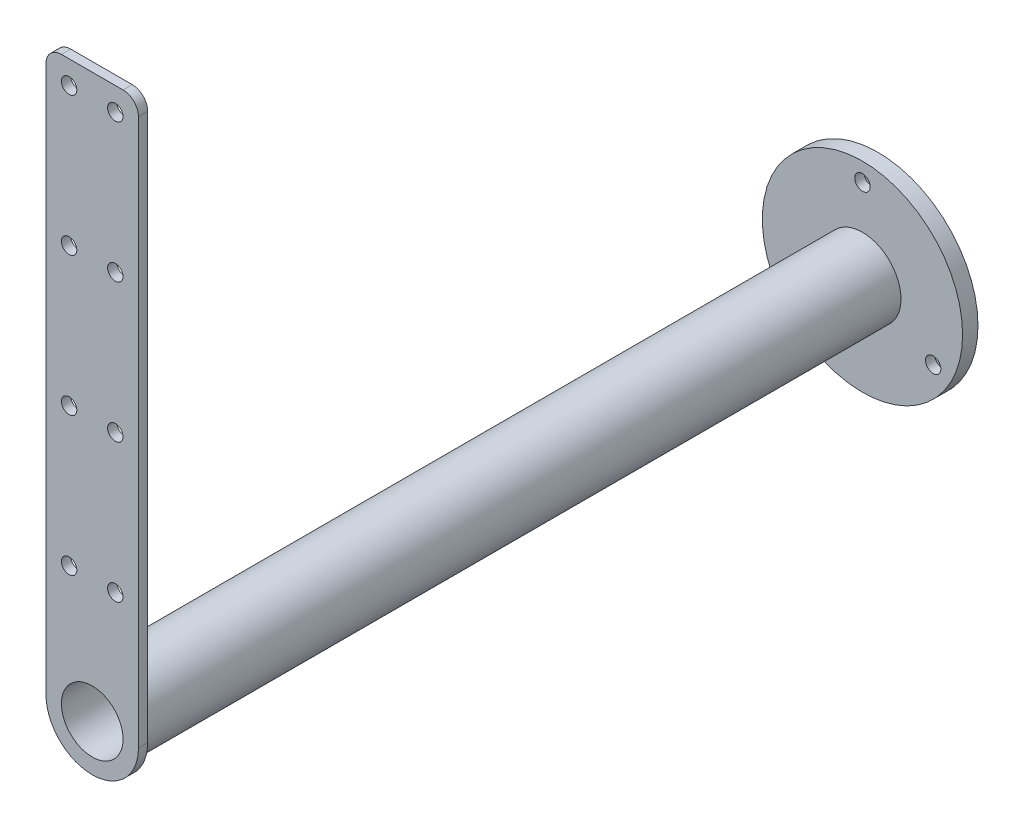
SolidWorks part; units mm, degrees
ref_plane "Front Plane" through (0, 0, 0) normal (0, 0, 1) x (1, 0, 0)
ref_plane "Top Plane" through (0, 0, 0) normal (0, 1, 0) x (1, 0, 0)
ref_plane "Right Plane" through (0, 0, 0) normal (1, 0, 0) x (0, 0, -1)
sketch "Sketch1" plane through (0, 0, 0) normal (0, 0, 1) x (1, 0, 0)
  circle A0 centre (0, 0) radius 65
  circle A1 centre (0, 0) radius 20
  dimension "D1" = 130
  dimension "D2" = 40
extrude "Boss-Extrude1" add sketch "Sketch1" along normal blind 10
sketch "Sketch2" plane through (0, 0, 10) normal (0, 0, 1) x (1, 0, 0)
  circle A0 centre (0, 0) radius 25
  circle A1 centre (0, 0) radius 20 construction
  circle A2 centre (0, 0) radius 20
  dimension "D1" = 50
extrude "Boss-Extrude2" add sketch "Sketch2" along normal blind 494
sketch "Sketch3" plane through (0, 0, 504) normal (0, 0, 1) x (1, 0, 0)
  line L0 (-30, 0) -> (-30, 365)
  line L1 (-30, 365) -> (30, 365)
  line L2 (30, 365) -> (30, 0)
  arc A0 (-30, 0) -> (30, 0) centre (0, 0) ccw
  circle A1 centre (0, 0) radius 20
  dimension "D1" = 60
  dimension "D2" = 365
extrude "Boss-Extrude3" add sketch "Sketch3" along normal blind 6
fillet "Fillet1" radius 10 2 edges at (-30, 365, 507) (30, 365, 507)
sketch "Sketch4" plane through (0, 0, 510) normal (0, 0, 1) x (1, 0, 0)
  line L0 (0, 365) -> (0, 386.1458) construction
  line L1 (20, 365) -> (-20, 365) construction
  circle A0 centre (-15, 350) radius 5
  circle A1 centre (15, 350) radius 5
  circle A2 centre (-15, 260) radius 5
  circle A3 centre (15, 260) radius 5
  circle A4 centre (-15, 170) radius 5
  circle A5 centre (15, 170) radius 5
  circle A6 centre (-15, 80) radius 5
  circle A7 centre (15, 80) radius 5
  dimension "D4" = 10
  dimension "D1" = 30
  dimension "D2" = 15
  dimension "D3" = 15
  dimension "D5" = 4
extrude "Cut-Extrude1" cut sketch "Sketch4" against normal blind 6
sketch "Sketch5" plane through (0, 0, 10) normal (0, 0, 1) x (1, 0, 0)
  circle A0 centre (0, 0) radius 53 construction
  circle A1 centre (0, 53) radius 5
  circle A2 centre (45.8993, -26.5) radius 5
  circle A3 centre (-45.8993, -26.5) radius 5
  point P11 (0, 0)
  dimension "D1" = 106
  dimension "D2" = 10
extrude "Cut-Extrude2" cut sketch "Sketch5" against normal blind 6
